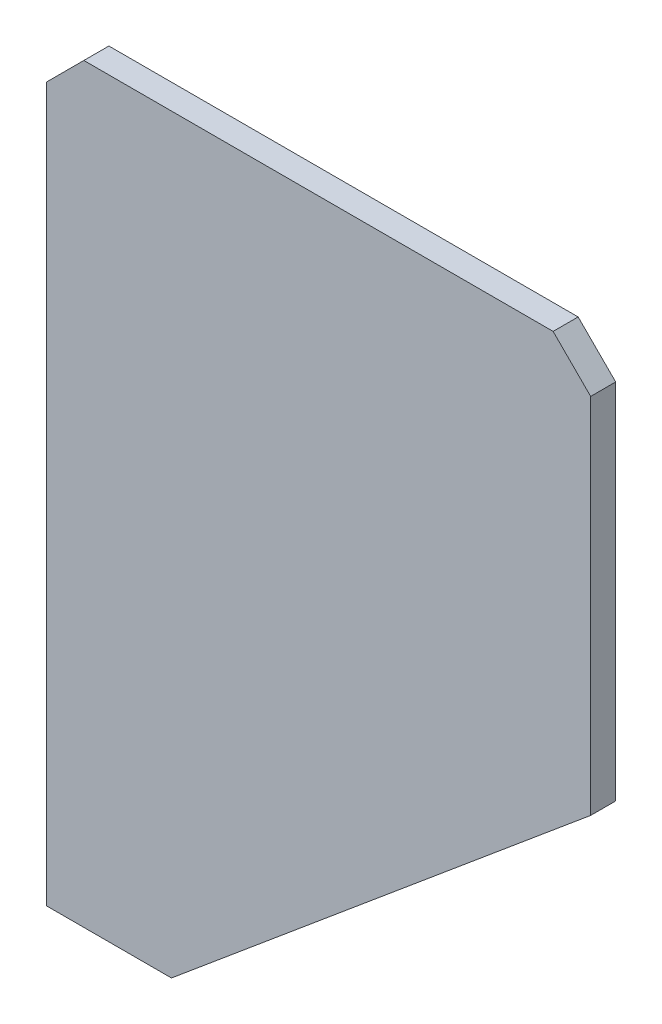
SolidWorks part; units mm, degrees
material "Q235-A"
ref_plane "前视基准面" through (0, 0, 0) normal (0, 0, 1) x (1, 0, 0)
ref_plane "上视基准面" through (0, 0, 0) normal (0, 1, 0) x (1, 0, 0)
ref_plane "右视基准面" through (0, 0, 0) normal (1, 0, 0) x (0, 0, -1)
sketch "草图1" plane through (0, 0, 0) normal (0, 0, 1) x (1, 0, 0)
  line L0 (0, 0) -> (43.5, 0)
  line L1 (43.5, 0) -> (43.5, -32)
  line L2 (43.5, -32) -> (10, -60)
  line L3 (10, -60) -> (0, -60)
  line L4 (0, -60) -> (0, 0)
  dimension "D1" = 43.5
  dimension "D2" = 60
  dimension "D3" = 32
  dimension "D4" = 10
extrude "凸台-拉伸1" add sketch "草图1" along normal blind 2
chamfer "倒角1" distance 3 angle 45 2 edges at (43.5, 0, 1) (0, 0, 1)
